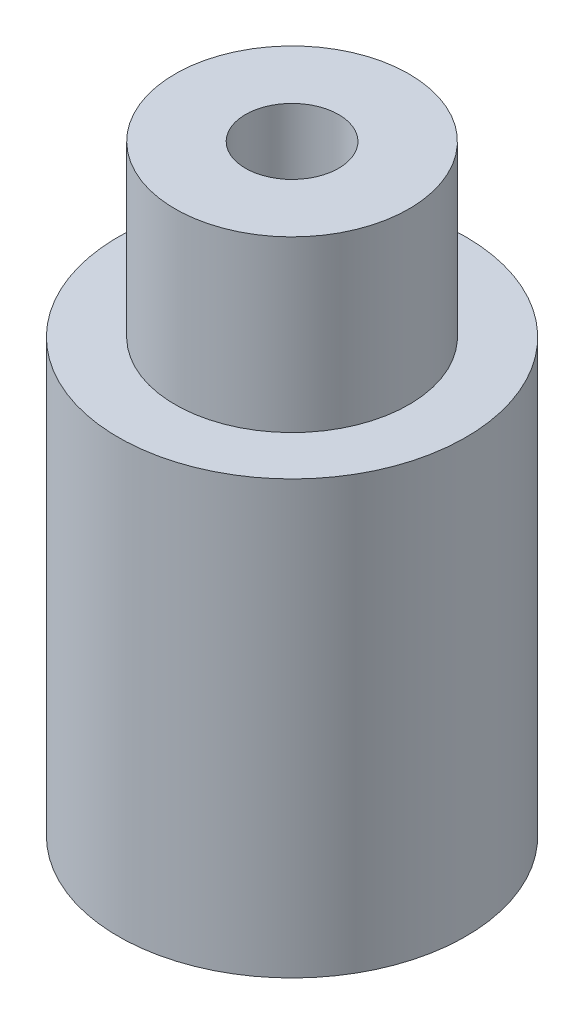
SolidWorks part; units mm, degrees
material "ABS"
ref_plane "Front Plane" through (0, 0, 0) normal (0, 0, 1) x (1, 0, 0)
ref_plane "Top Plane" through (0, 0, 0) normal (0, 1, 0) x (1, 0, 0)
ref_plane "Right Plane" through (0, 0, 0) normal (1, 0, 0) x (0, 0, -1)
sketch "Sketch1" plane through (0, 0, 0) normal (0, 0, 1) x (1, 0, 0)
  line L0 (-0.55, -1.5) -> (-2.05, -1.5)
  line L1 (-2.05, -1.5) -> (-2.05, 3.6)
  line L2 (-2.05, 3.6) -> (-1.38, 3.6)
  line L3 (-1.38, 3.6) -> (-1.38, 5.6)
  line L4 (-1.38, 5.6) -> (-0.55, 5.6)
  line L5 (-0.55, 5.6) -> (-0.55, -1.5)
  line L6 (0, -0.7316) -> (0, 5.7628) construction
  line L10 (-2.1, -1.5) -> (2.1, -1.5) construction
  dimension "D1" = 1.1
  dimension "D3" = 4.1
revolve "Revolve1" add sketch "Sketch1" angle 360 about L6
